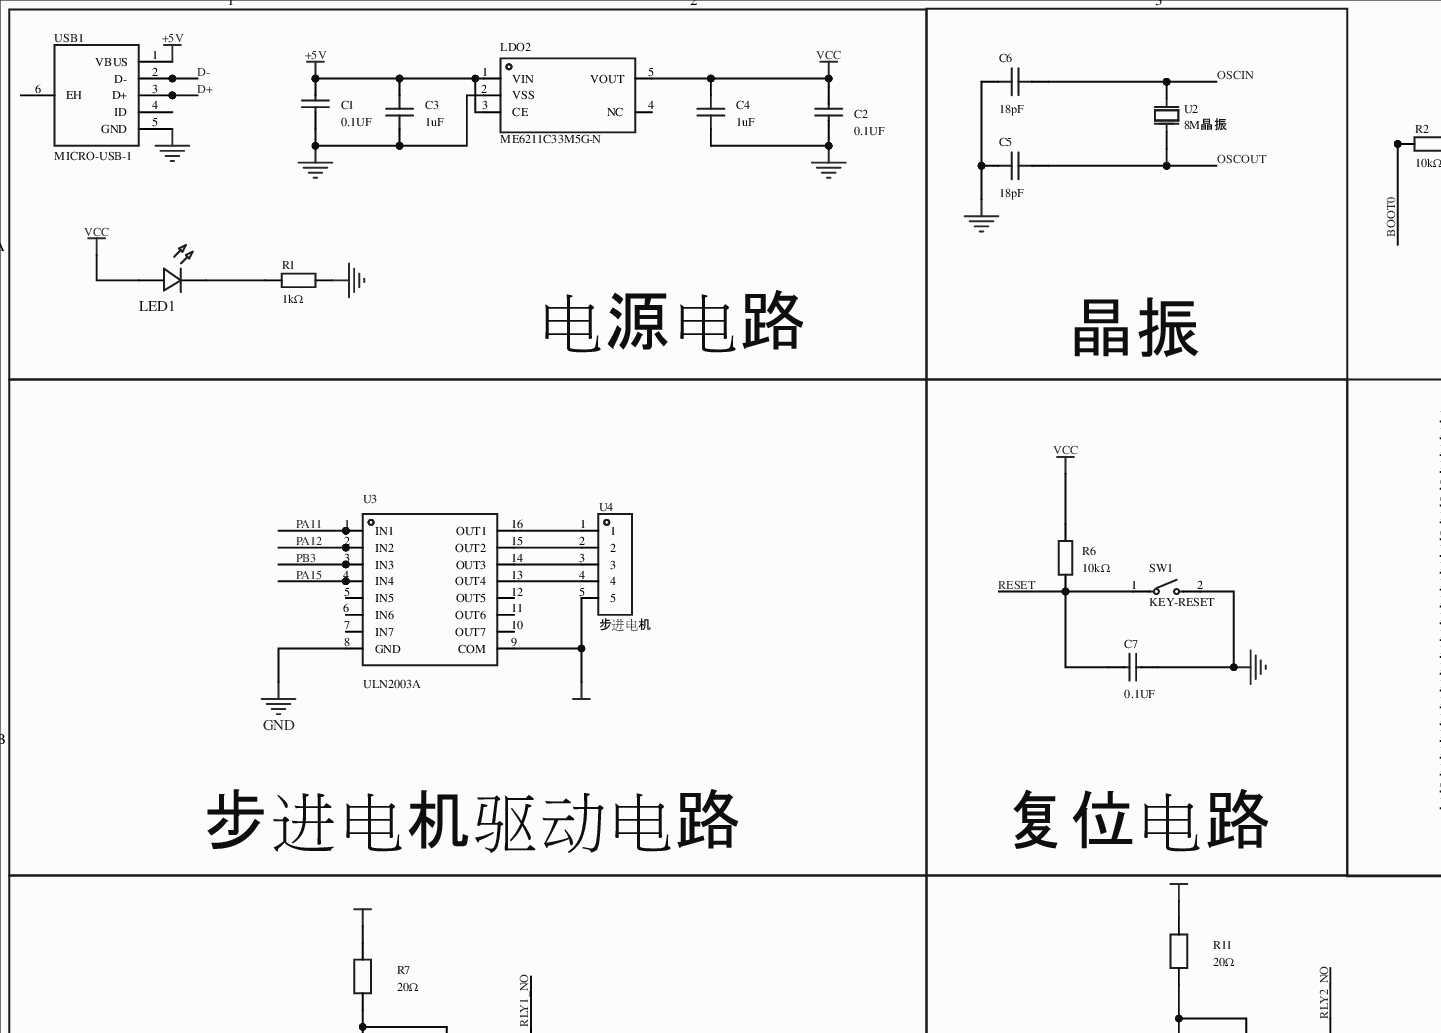
[diagram p0: MISC51317-3.schdoc, top left]
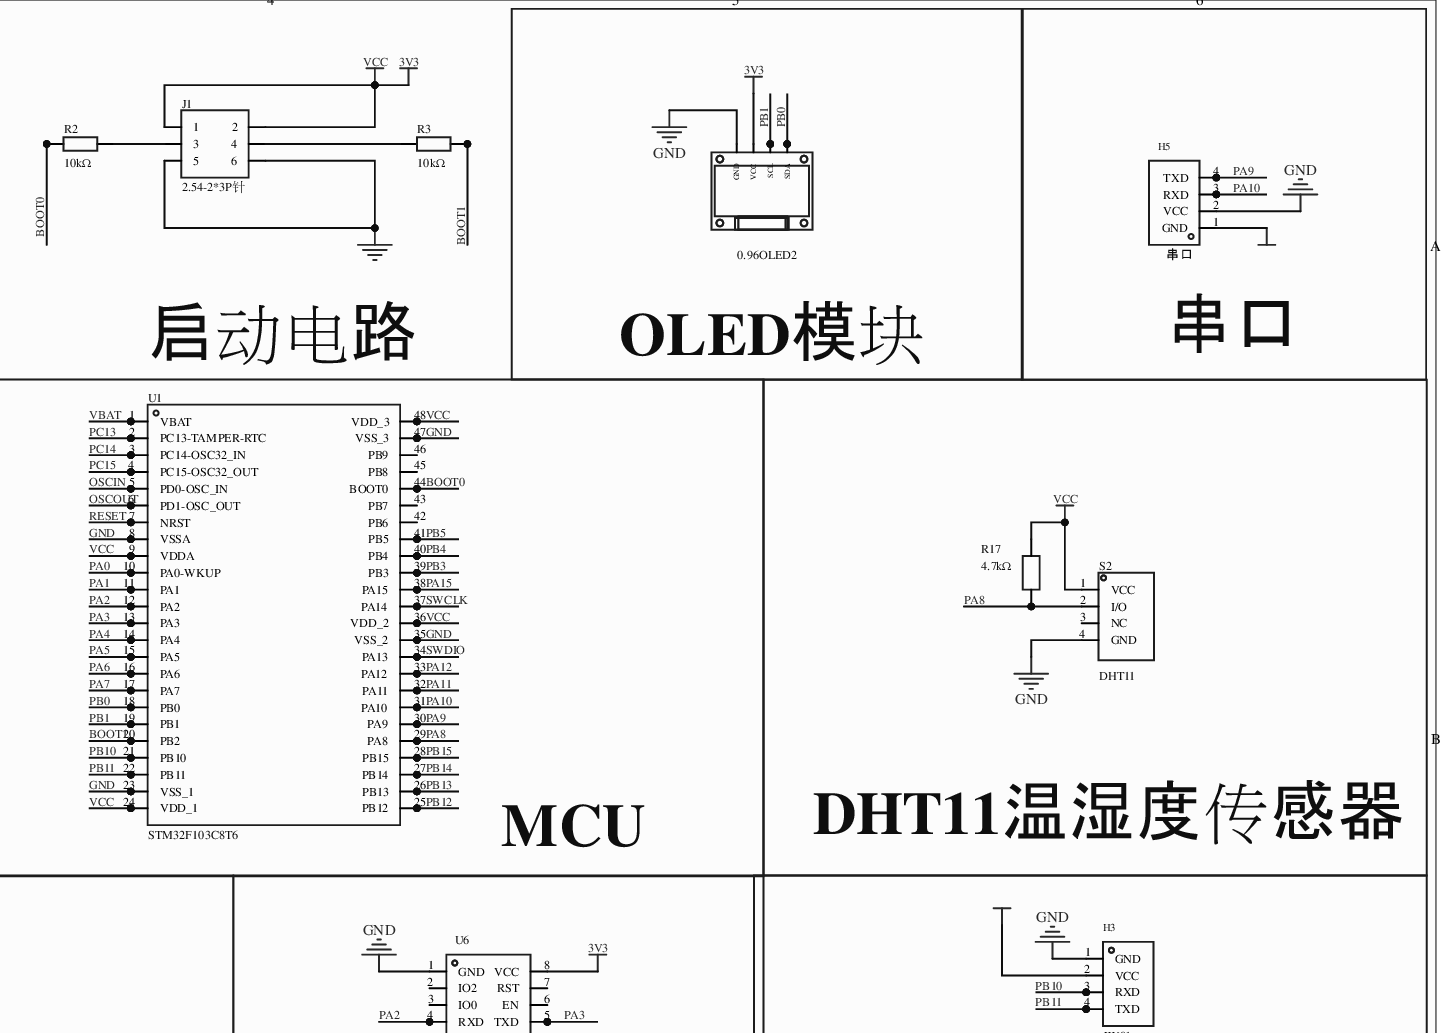
[diagram p1: MISC51317-3.schdoc, top right]
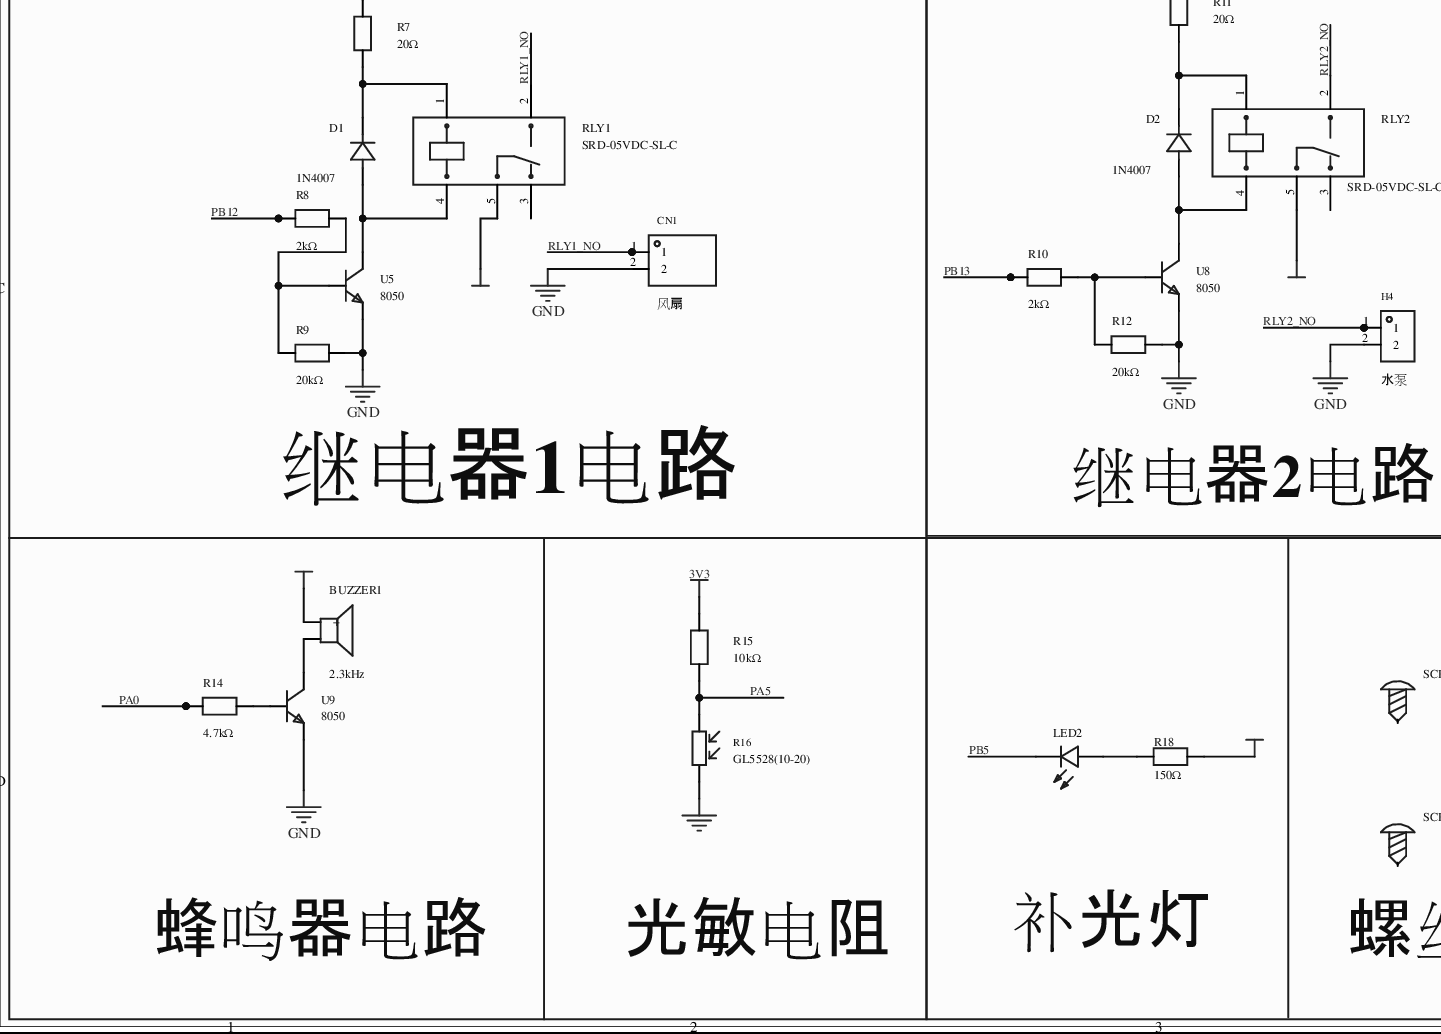
[diagram p2: MISC51317-3.schdoc, bottom left]
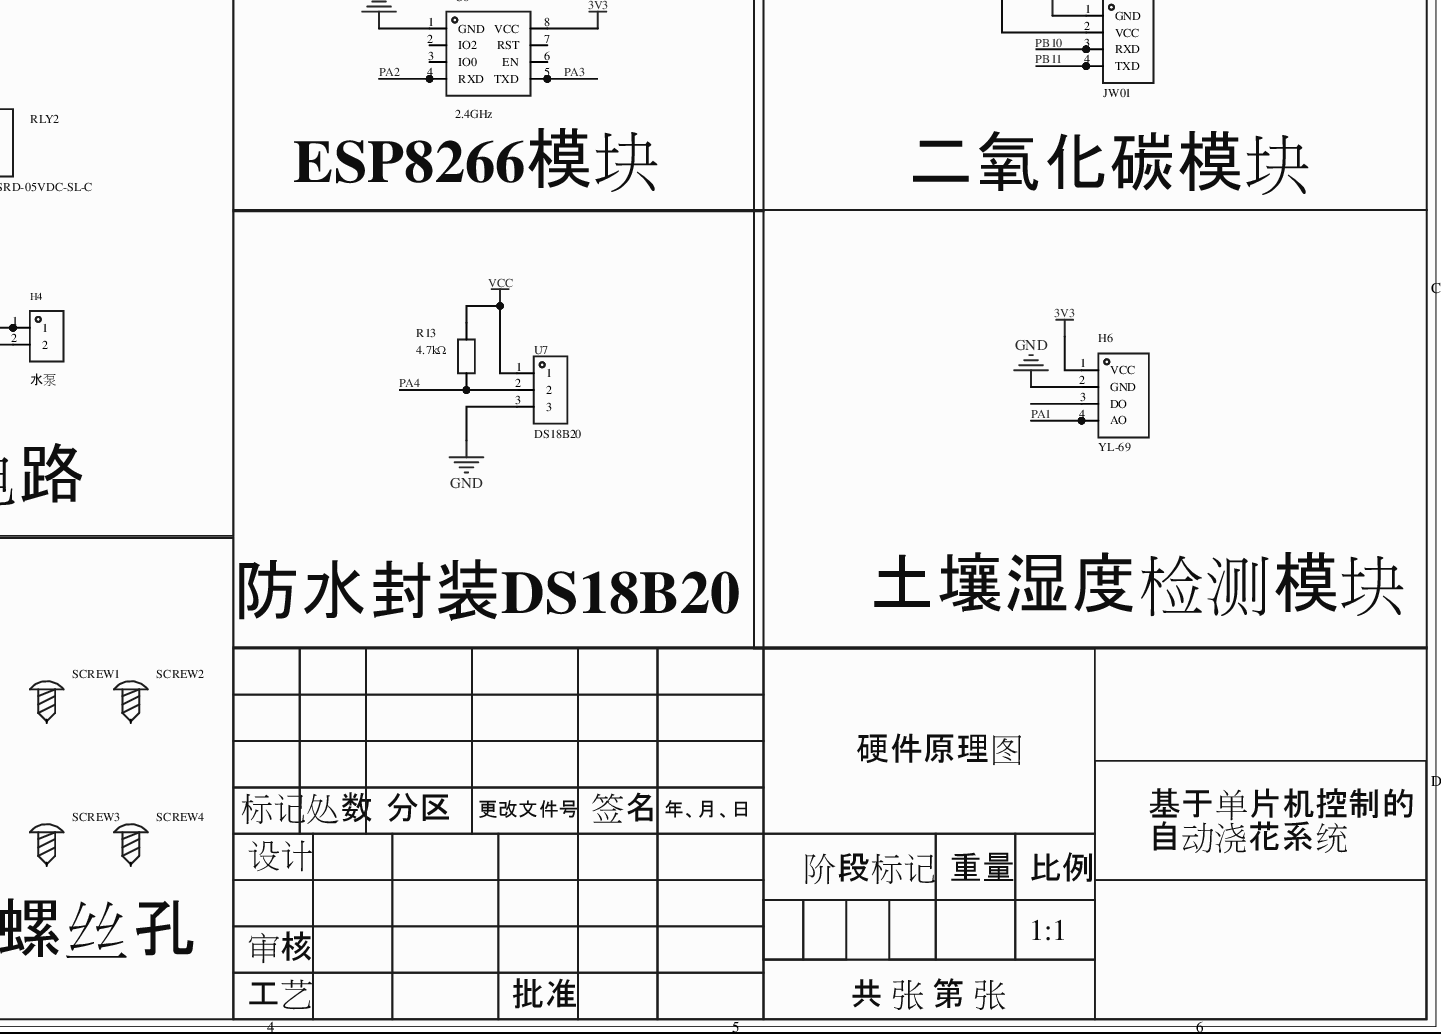
[diagram p3: MISC51317-3.schdoc, bottom right]
# Altium project MISC51317-2.PrjPcb
1 sheet, 54 parts. Net scope: global (net labels, ports and power ports of the same name join across sheets).
Board file: MISC51317.pcbdoc

## Sheet MISC51317-3.schdoc
size 420 x 297 mm; Version: V1.0; @Project Name: MISC51317; @Update Date: 2026-04-15; @Create Date: 2026-04-15; @Board Name: MISC51317; @Create Time: 10:52:34; @Page Count: 1; @Page No: 1; @Schematic Name: MISC51317; @Update Time: 10:52:34; Size: A4

### Parts
0.96OLED2  (no value)  [oled-th_l27.8-w27.2-p2.54_c9900033791]
BUZZER1  2.3kHz  [BUZ-TH_BD12.0-P7.60-D0.6-FD]
C1  0.1UF  [C0603]
C2  0.1UF  [C0603]
C3  1uF  [C0603]
C4  1uF  [C0603]
C5  18pF  [C0603]
C6  18pF  [C0603]
C7  0.1UF  [C0603]
CN1  风扇  [CONN-TH_B2B-XH-A-LF-SN]
D1  1N4007  [DO-41_BD2.4-L4.7-P8.70-D0.8-RD]
D2  1N4007  [DO-41_BD2.4-L4.7-P8.70-D0.8-RD]
H3  JW01  [HDR-TH_4P-P2.54-V-M]
H4  水泵  [HDR-TH_2P-P2.54-V-M]
H5  串口  [HDR-TH_4P-P2.54-V-M]
H6  YL-69  [HDR-TH_4P-P2.54-V-F]
J1  2.54-2*3P针  [HDR-TH_6P-P2.54-V-M-R2-C3-S2.54-1]
LDO2  ME6211C33M5G-N  [SOT-23-5_L3.0-W1.7-P0.95-LS2.8-BL]
LED1  (no value)  [LED_0603]
LED2  (no value)  [LED-TH_BD5.9-P2.54-RD]
R1  1kΩ  [R0603]
R2  10kΩ  [R0603]
R3  10kΩ  [R0603]
R6  10kΩ  [R0603]
R7  20Ω  [RES-TH_BD2.3-L6.5-P10.50-D0.5]
R8  2kΩ  [RES-TH_BD2.3-L6.5-P10.50-D0.5]
R9  20kΩ  [RES-TH_BD2.3-L6.5-P10.50-D0.5]
R10  2kΩ  [RES-TH_BD2.3-L6.5-P10.50-D0.5]
R11  20Ω  [RES-TH_BD2.3-L6.5-P10.50-D0.5]
R12  20kΩ  [RES-TH_BD2.3-L6.5-P10.50-D0.5]
R13  4.7kΩ  [RES-TH_BD2.3-L6.5-P10.50-D0.5]
R14  4.7kΩ  [RES-TH_BD2.3-L6.5-P10.50-D0.5]
R15  10kΩ  [RES-TH_BD2.3-L6.5-P10.50-D0.5]
R16  GL5528(10-20)  [RES-TH_L5.1-W4.3-P3.40-D0.5]
R17  4.7kΩ  [RES-TH_BD2.3-L6.5-P10.50-D0.5]
R18  150Ω  [RES-TH_BD2.3-L6.5-P10.50-D0.5]
RLY1  SRD-05VDC-SL-C  [RELAY-TH_SRD-XXVDC-XL-C]
RLY2  SRD-05VDC-SL-C  [RELAY-TH_SRD-XXVDC-XL-C]
S2  DHT11  [SENSOR-TH_DHT11-1]
SCREW1  (no value)  [M2螺丝]
SCREW2  (no value)  [M2螺丝]
SCREW3  (no value)  [M2螺丝]
SCREW4  (no value)  [M2螺丝]
SW1  KEY-RESET  [SW-SMD_L6.0-W3.3-LS8.0]
U1  STM32F103C8T6  [LQFP-48_L7.0-W7.0-P0.50-LS9.0-BL]
U2  8M晶振  [HC-49S_L11.5-W4.7-P4.88]
U3  ULN2003A  [DIP-16_L20.0-W6.4-P2.54-LS7.6-BL]
U4  步进电机  [CONN-TH_5P-P2.50_ZHOURI_XH-5PA]
U5  8050  [TO-92-3_L4.8-W3.7-P2.54-R]
U6  2.4GHz  [WIFIM-TH_8P-L24.7-W14.4-P2.54]
U7  DS18B20  [CONN-TH_3P-P5.00_KF301-5.0-3P]
U8  8050  [TO-92-3_L4.8-W3.7-P2.54-R]
U9  8050  [TO-92-3_L4.8-W3.7-P2.54-R]
USB1  MICRO-USB-1  [MICRO-USB-SMD_C9900008946]

### Blocks framed on the sheet
电源电路: C1-C4 LDO2 LED1 R1 USB1
晶振: C5 C6 U2
OLED模块: 0.96OLED2
串口: H5
步进电机驱动电路: U3 U4
复位电路: C7 R6 SW1
DHT11温湿度传感器: R17 S2
继电器1电路: CN1 D1 R7-R9 RLY1 U5
继电器2电路: D2 H4 R10-R12 RLY2 U8
二氧化碳模块: H3
土壤湿度检测模块: H6
蜂鸣器电路: BUZZER1 R14 U9
光敏电阻: R15 R16

### Nets
+5V: C1.2 C3.2 LDO2.1(VIN) LDO2.3(CE) USB1.1(VBUS)
GND: 0.96OLED2.1(GND) C1.1 C2.1 C3.1 C4.1 C5.2 C6.1 C7.2 CN1.2 H3.1(GND) H4.2 H5.2(VCC) H6.2(GND) J1.5 J1.6 LDO2.2(VSS) R1.2 R9.2 R12.2 R16.2 S2.4(GND) SW1.2 U1.8(VSSA) U1.23(VSS_1) U1.35(VSS_2) U1.47(VSS_3) U3.8(GND) U5.3(E) U6.1(GND) U7.3 U8.3(E) U9.3(E) USB1.5(GND)
3V3: 0.96OLED2.2(VCC) BUZZER1.1(+) C2.2 C4.2 H3.2(VCC) H5.1(GND) H6.1(VCC) J1.1 J1.2 LDO2.5(VOUT) LED1.2(A) R6.2 R7.2 R11.2 R13.2 R15.2 R17.2 R18.2 RLY1.5 RLY2.5 S2.1(VCC) U1.9(VDDA) U1.24(VDD_1) U1.36(VDD_2) U1.48(VDD_3) U3.9(COM) U4.5 U6.8(VCC) U7.1  [also labelled VCC]
BOOT0: R2.1 U1.44(BOOT0)
BOOT1: R3.2 U1.20(PB2)
D+: USB1.3(D+)
D-: USB1.2(D-)
OSCIN: C6.2 U1.5(PD0-OSC_IN) U2.1(OSC1)
OSCOUT: C5.1 U1.6(PD1-OSC_OUT) U2.2(OSC2)
PA0: R14.1 U1.10(PA0-WKUP)
PA1: H6.4(AO) U1.11(PA1)
PA2: U1.12(PA2) U6.4(RXD)
PA3: U1.13(PA3) U6.5(TXD)
PA4: R13.1 U1.14(PA4) U7.2
PA5: R15.1 R16.1 U1.15(PA5)
PA6: U1.16(PA6)
PA7: U1.17(PA7)
PA8: R17.1 S2.2(I/O) U1.29(PA8)
PA9: H5.4(TXD) U1.30(PA9)
PA10: H5.3(RXD) U1.31(PA10)
PA11: U1.32(PA11) U3.1(IN1)
PA12: U1.33(PA12) U3.2(IN2)
PA15: U1.38(PA15) U3.4(IN4)
PB0: 0.96OLED2.4(SDA) U1.18(PB0)
PB1: 0.96OLED2.3(SCL) U1.19(PB1)
PB3: U1.39(PB3) U3.3(IN3)
PB4: U1.40(PB4)
PB5: LED2.1(C) U1.41(PB5)
PB10: H3.3(RXD) U1.21(PB10)
PB11: H3.4(TXD) U1.22(PB11)
PB12: R8.1 U1.25(PB12)
PB13: R10.1 U1.26(PB13)
PB14: U1.27(PB14)
PB15: U1.28(PB15)
PC13: U1.2(PC13-TAMPER-RTC)
PC14: U1.3(PC14-OSC32_IN)
PC15: U1.4(PC15-OSC32_OUT)
RESET: C7.1 R6.1 SW1.1 U1.7(NRST)
RLY1_NO: CN1.1 RLY1.2
RLY2_NO: H4.1 RLY2.2
SWCLK: U1.37(PA14)
SWDIO: U1.34(PA13)
VBAT: U1.1(VBAT)
NetBUZZER1_2: BUZZER1.2 U9.1(C)
NetD1_1: D1.1(K) R7.1 RLY1.1
NetD1_2: D1.2(A) RLY1.4 U5.1(C)
NetD2_1: D2.1(K) R11.1 RLY2.1
NetD2_2: D2.2(A) RLY2.4 U8.1(C)
NetJ1_3: J1.3 R2.2
NetJ1_4: J1.4 R3.1
NetLED1_1: LED1.1(C) R1.1
NetLED2_2: LED2.2(A) R18.1
NetR8_2: R8.2 R9.1 U5.2(B)
NetR10_2: R10.2 R12.1 U8.2(B)
NetR14_2: R14.2 U9.2(B)
NetU3_13: U3.13(OUT4) U4.4
NetU3_14: U3.14(OUT3) U4.3
NetU3_15: U3.15(OUT2) U4.2
NetU3_16: U3.16(OUT1) U4.1

Not connected (* = marked no-connect by the designer): H6 3(DO); LDO2 4(NC)*; RLY1 3*; RLY2 3*; S2 3(NC); SCREW1 1; SCREW2 1; SCREW3 1; SCREW4 1; U1 42(PB6)* 43(PB7)* 45(PB8)* 46(PB9)*; U3 5(IN5)* 6(IN6)* 7(IN7)* 10(OUT7)* 11(OUT6)* 12(OUT5)*; U6 2(IO2)* 3(IO0)* 6(EN)* 7(RST)*; USB1 4(ID)* 6(EH)*

### Notes on the sheet
- (near U1) 启动电路
- MCU
- (near U6) ESP8266模块
- 防水封装DS18B20
- 硬件原理图
- 基于单片机控制的
  自动浇花系统
- 标记
- 设计
- 处数
- 分区
- 更改文件号
- 签名
- 年、月、日
- 阶段标记
- 重量
- 比例
- 补光灯
- 螺丝孔
- 审核
- 1:1
- 工艺
- 批准
- 共 张 第 张

### Library data of the parts
0.96OLED2 = 0.96OLED模块_4P: 3D Model: 79c000fdb68d45a296c2e9bedf4f9055; 3D Model Transform: 1393.69792,1318.895,0,0,0,0,0,-560.079,-137.795; ConvertToPcb: yes; ModelName: 0.96OLED_4P; Device: 0.96OLED模块_4P; Symbol: 0.96OLED模块_4P; Supplier Footprint: 插件; FootprintName: oled-th_l27.8-w27.2-p2.54_c9900033791; AddInBom: yes
BUZZER1 = TMB12A05_C96093: 驱动方式:有源(内含驱动线路);构造类型:电磁式;额定电压:5V;频率:2.3kHz;声压(SPL):85dB@5V,10cm;; Manufacturer: 华能; 3D Model: 16ab50e14c5b4f2c986c135bdba60e37; 3D Model Transform: 472.44,472.176,0,90,0,0,-0.787,0,-177.165; Technology Type: 电磁式; Rated Voltage: 5V; Operating Voltage: 4V~8V; AddInBom: yes; ModelName: BUZ-TH_D12.0-H9.5-P7.60; Device: TMB12A05_C96093; Symbol: TMB12A05; LCSC Part Name: TMB12A05; Supplier Part: C96093; Manufacturer Part: TMB12A05; Supplier Footprint: 插件,D=12mm; JLCPCB Part Class: Extended Part; Datasheet: https://atta.szlcsc.com/upload/public/pdf/source/20170522/1495448324811.pdf; Supplier: LCSC; Oscillator Circuit: 有源(内含驱动线路); Value: 2.3kHz; Sound Pressure Level (SPL): 85dB@5V,10cm; Diameter (φD): 12mm; Height: 9.8mm; FootprintName: BUZ-TH_BD12.0-P7.60-D0.6-FD; ConvertToPcb: yes
C1 C2 = CAPCER0.1UF16VX5R0603,CAPCER0.1UF25VX5R0603,CAPCER0.1UF16VX7R0603: AddInBom: yes; ModelId: ac125912035d415993ca9572d50418b10819f05c4eef4c71ace90d822a990e87; ModelName: C0603_L1.6-W0.8-H0.8; ModelTransform: 62.992,31.496,0,0,0,0,0,0,0; Device: CAPCER0.1UF16VX5R0603,CAPCER0.1UF25VX5R0603,CAPCER0.1UF16VX7R0603; Symbol: CAPCER0.1UF16VX5R0603,CAPCER0.1UF25VX5R0603,CAPCER0.1UF16VX7R0603; Manufacturer Part: 0.1UF; FootprintName: C0603; LCSC Part Name: CAPCER0.1UF16VX5R0603,CAPCER0.1UF25VX5R0603,CAPCER0.1UF16VX7R0603; SupplierPart: C9900012833; Supplier Footprint: C0603; JLCPCB Part Class: Extended Part; Supplier: LCSC; ConvertToPcb: yes
C3 C4 = TMK107B7105MA-T: 容值:1uF;精度:±20%;额定电压:25V;温度系数:X7R;; Manufacturer: TAIYO YUDEN(太诱); AddInBom: yes; Tolerance: ±20%; Voltage Rating: 25V; Temperature Coefficient: X7R; ModelId: ac125912035d415993ca9572d50418b10819f05c4eef4c71ace90d822a990e87; ModelName: C0603_L1.6-W0.8-H0.8; ModelTransform: 62.992,31.496,0,0,0,0,0,0,0; Device: TMK107B7105MA-T; Symbol: TMK107B7105MA-T; FootprintName: C0603; LCSC Part Name: MSAST168SB7105MTNA01 1uF ±20% 25V; SupplierPart: C2180866; ManufacturerPart: TMK107B7105MA-T; Supplier Footprint: 0603; JLCPCB Part Class: Extended Part; Datasheet: https://item.szlcsc.com/datasheet/TMK107B7105MA-T/2272933.html; Supplier: LCSC; ConvertToPcb: yes; Value: 1uF
C5 C6 = C1608C0G1H180J080AA: 容值:18pF;精度:±5%;额定电压:50V;材质(温度系数):C0G;; Manufacturer: TDK; AddInBom: yes; Tolerance: ±5%; Voltage Rated: 50V; Temperature Coefficient: C0G; ModelId: ac125912035d415993ca9572d50418b10819f05c4eef4c71ace90d822a990e87; ModelName: C0603_L1.6-W0.8-H0.8; ModelTransform: 62.992,31.496,0,0,0,0,0,0,0; Device: C1608C0G1H180J080AA; Symbol: C1608C0G1H180J080AA; FootprintName: C0603; LCSC Part Name: 18pF ±5% 50V; SupplierPart: C3902597; ManufacturerPart: C1608C0G1H180J080AA; Supplier Footprint: 0603; JLCPCB Part Class: Extended Part; Datasheet: https://atta.szlcsc.com/upload/public/pdf/source/20230606/A83975C7E70EF5AFCD4A17254ABD78F2.pdf; Supplier: LCSC; ConvertToPcb: yes; Value: 18pF
C7 = CAPCER0.1UF16VX5R0603,CAPCER0.1UF25VX5R0603,CAPCER0.1UF16VX7R0603: 3D Model: ac125912035d415993ca9572d50418b10819f05c4eef4c71ace90d822a990e87; 3D Model Transform: 62.992,31.496,0,0,0,0,0,0,0; AddInBom: yes; ModelName: C0603_L1.6-W0.8-H0.8; Device: CAPCER0.1UF16VX5R0603,CAPCER0.1UF25VX5R0603,CAPCER0.1UF16VX7R0603; Symbol: CAPCER0.1UF16VX5R0603,CAPCER0.1UF25VX5R0603,CAPCER0.1UF16VX7R0603; LCSC Part Name: CAPCER0.1UF16VX5R0603,CAPCER0.1UF25VX5R0603,CAPCER0.1UF16VX7R0603; Supplier Part: C9900012833; Manufacturer Part: 0.1UF; Supplier Footprint: C0603; JLCPCB Part Class: Extended Part; Supplier: LCSC; FootprintName: C0603; ConvertToPcb: yes
CN1 = B2B-XH-A(LF)(SN): 参考系列:XH;间距:2.5mm;插针结构:1x2P;排数:1;每排PIN数:2;行距:-;安装方式:-;触头材质:黄铜;; Manufacturer: JST; 3D Model: 2cd591bdb98c4759a6cba2f4f7745e41; 3D Model Transform: 295.275,224.44837,0,180,0,0,0,18.701,-98.425; Reference Series: XH; Pitch: 2.5mm; Pins Structure: 1x2P; Number of PINs Per Row: 2; AddInBom: yes; ModelName: XH2.5-2A; Device: B2B-XH-A(LF)(SN); Symbol: B2B-XH-A (LF)(SN); Manufacturer Part: 风扇; LCSC Part Name: 系列:XH 间距:2.5mm 1x2P; Supplier Footprint: 插件,P=2.5mm; Datasheet: https://atta.szlcsc.com/upload/public/pdf/source/20180928/C265283_F9DFEEBDB2CF642B6BDFAB4B77BD2680.pdf; Number of Rows: 1; Row Spacing: -; Mounting Style: -; Contact Material: 黄铜; Supplier: LCSC; Supplier Part: C158012; JLCPCB Part Class: 扩展库; FootprintName: CONN-TH_B2B-XH-A-LF-SN; ConvertToPcb: yes
D1 D2 = 1N4007_C2985028: 直流反向耐压(Vr):1kV;平均整流电流(Io):1A;正向压降(Vf):1V@1A;; Manufacturer: GOODWORK(固得沃克); 3D Model: 6de1e9b71a0d4751b4e9df530304c1a3; 3D Model Transform: 374.015,94.428,0,0,0,0,0,0,-137.795; Reverse Voltage (Vr): 1kV; Average Rectified Current (Io): 1A; Forward Voltage (Vf@If): 1V@1A; AddInBom: yes; ModelName: DO-41_D2.4-L4.7-P8.70; Device: 1N4007_C2985028; Symbol: 1N4007_C2985028; LCSC Part Name: 1kV 1A 1V@1A; Supplier Part: C2985028; Manufacturer Part: 1N4007; Supplier Footprint: DO-41; JLCPCB Part Class: 扩展库; Datasheet: https://atta.szlcsc.com/upload/public/pdf/source/20210723/C2848669_ECFE0BC1B34B7BAAA686846FF0F306A7.pdf; Supplier: LCSC; FootprintName: DO-41_BD2.4-L4.7-P8.70-D0.8-RD; ConvertToPcb: yes
H3 H5 = PZ254V-11-04P: 排数:单排;总PIN位数:4P;间距:2.54mm;插针结构:1x4P;行距:-;安装类型:直插;圆针/方针:方针;额定电流:3A;额定电压:250V;配合针长度:6mm;塑高:2.5mm;端接针长度:3mm;触头材质:-;工作温度范围:-40℃~+105℃;颜色:黑色;; Manufacturer: XFCN(兴飞); Symbol: PZ254V-11-04P_C2691448; 3D Model: 112f4d05e8d64e99ab9a333894bea4f9; 3D Model Transform: 399.999,104.7242,0,0,0,0,0,0,-118.11; Pitch: 2.54mm; Pin Structure: 1x4P; Circluar Pins/Square Pins: 方针; Current Rating (Max): 3A; Voltage Rating (Max): 250V; AddInBom: yes; ModelName: HDR-TH_4P-P2.54-M-LI-1X4P; Device: PZ254V-11-04P; LCSC Part Name: 2.54mm 1x4P 直插 方针; Supplier Part: C2691448; Supplier Footprint: 插件,P=2.54mm; JLCPCB Part Class: 扩展库; Datasheet: https://atta.szlcsc.com/upload/public/pdf/source/20200309/C492403_F9F19131791D08044AD4F84F8E751A34.pdf; Supplier: LCSC; Number of Rows: 单排; Number of Pins: 4P; Row Spacing: -; Mounting Type: 直插; Length of Mating Pin: 6mm; Insulation Height: 2.5mm; Length of End Connection Pin: 3mm; Contact Material: -; Operating Temperature Range: -40℃~+105℃; Color: 黑色; FootprintName: HDR-TH_4P-P2.54-V-M; ConvertToPcb: yes
  H3: Manufacturer Part: JW01
  H5: Manufacturer Part: 串口
H4 = PZ254V-11-02P: 排数:单排;总PIN位数:2P;间距:2.54mm;插针结构:1x2P;行距:-;安装类型:直插;圆针/方针:方针;额定电流:-;额定电压:-;配合针长度:6mm;塑高:2.5mm;端接针长度:3mm;触头材质:黄铜;触头镀层:-;工作温度范围:-40℃~+105℃;颜色:黑色;; Manufacturer: XFCN(兴飞); 3D Model: e35305ec3aa84b66b849f914b715e73f; 3D Model Transform: 200,100,0,0,0,0,0,0,-118.11; Pitch: 2.54mm; Pin Structure: 1x2P; Circluar Pins/Square Pins: 方针; AddInBom: yes; ModelName: HDR2.54-M-LI-1X2P; Device: PZ254V-11-02P; Symbol: PZ254V-11-02P; Manufacturer Part: 水泵; LCSC Part Name: 2.54mm 1x2P 直插 方针; Supplier Footprint: 插件,P=2.54mm; Datasheet: https://atta.szlcsc.com/upload/public/pdf/source/20200309/C492401_A812433581A9B211A7FFA413ADDFF0E5.pdf; Number of Rows: 单排; Number of Pins: 2P; Row Spacing: -; Mounting Type: 直插; Current Rating (Max): -; Voltage Rating (Max): -; Length of Mating Pin: 6mm; Insulation Height: 2.5mm; Length of End Connection Pin: 3mm; Contact Material: 黄铜; Contact Plating: -; Operating Temperature Range: -40℃~+105℃; Color: 黑色; Supplier: LCSC; Supplier Part: C492401; JLCPCB Part Class: 扩展库; FootprintName: HDR-TH_2P-P2.54-V-M; ConvertToPcb: yes
H6 = PM254V-11-04-H85: 排数:单排;总孔位数:4P;间距:2.54mm;插孔结构:1x4P;行距:-;安装类型:直插;塑高:-;触头材质:黄铜;触头镀层:-;; Manufacturer: XFCN(兴飞); 3D Model: 57daaad411c24bd7bd5d06edf5c4d16b; 3D Model Transform: 415.7472,98.425,0,0,0,0,0,0,-118.11; Number of Holes: 4P; Pitch: 2.54mm; Holes Structure: 1x4P; AddInBom: yes; ModelName: HDR-TH_4P-P2.54-F-LI-1X4P; Device: PM254V-11-04-H85; Symbol: PM254V-11-04-H85; Manufacturer Part: YL-69; LCSC Part Name: 间距:2.54mm 1x4P 直插; Supplier Part: C541851; Supplier Footprint: 插件,P=2.54mm; JLCPCB Part Class: 扩展库; Datasheet: https://atta.szlcsc.com/upload/public/pdf/source/20200518/C541849_85853D71FC67C51915A806977A588FDA.pdf; Supplier: LCSC; Number of Rows: 单排; Row Spacing: -; Mounting Type: 直插; Insulation Height: -; Contact Material: 黄铜; Contact Plating: -; FootprintName: HDR-TH_4P-P2.54-V-F; ConvertToPcb: yes
J1 = 2.54-2*3P针: 插针结构:-;间距:2.54mm;行距:2.54mm;圆针/方针:-;安装方式:直插;排数:双排;总PIN位数:6P;额定电流:-;额定电压:-;配合针长度:-;塑高:-;触头材质:-;触头镀层:-;颜色:黑色;; Manufacturer: BOOMELE(博穆精密); Symbol: Header-Male-2.54_2x3; AddInBom: yes; Pitch: 2.54mm; ModelId: fd1b55b786fb415ca65c4187088147b70819f05c4eef4c71ace90d822a990e87; ModelName: HDR2.54-M-LI-2x3P; ModelTransform: 299.9994,200,0,0,0,0,0,0,-118.11; Device: 2.54-2*3P针; FootprintName: HDR-TH_6P-P2.54-V-M-R2-C3-S2.54-1; LCSC Part Name: 间距:2.54mm 直插; SupplierPart: C65114; ManufacturerPart: 2.54-2*3P针; Supplier Footprint: 插件,P=2.54mm; JLCPCB Part Class: Extended Part; Supplier: LCSC; ConvertToPcb: yes; Pin Structure: -; Row Spacing: 2.54mm; Circluar Pins/Square Pins: -; Mounting Type: 直插; Number of Rows: 双排; Number of Pins: 6P; Current Rating: -; Voltage Rating (Max): -; Length of Mating Pin: -; Insulation Height: -; Contact Material: -; Contact Plating: -; Color: 黑色
LDO2 = ME6211C33M5G-N: 输出类型:固定;工作电压:6V;输出电压:3.3V;输出电流:500mA;电源纹波抑制比(PSRR):70dB@(1kHz);输出极性:正极;; Manufacturer: MICRONE(南京微盟); AddInBom: yes; Output Type: 固定; Voltage - Supply: 6V; Output Voltage: 3.3V; Output Current: 500mA; Voltage Dropout: 120mV@(100mA); standby current: 60uA; Noise: 50uVrms; Output Configuration: 正极; Number of Outputs: 1; ModelId: 0a2a1b8f50944f73965918ad6e5fe1670819f05c4eef4c71ace90d822a990e87; ModelName: SOT-23-5_L2.9-W1.6-H1.1-LS2.8-P0.95; ModelTransform: 118.60433,114.173,0,90,0,0,0.0005,0.0005,0; Device: ME6211C33M5G-N; Symbol: ME6211C33M5G-N; FootprintName: SOT-23-5_L3.0-W1.7-P0.95-LS2.8-BL; LCSC Part Name: 输入6V 输出3.3V 500mA; SupplierPart: C82942; ManufacturerPart: ME6211C33M5G-N; Supplier Footprint: SOT-23-5; JLCPCB Part Class: Extended Part; Datasheet: https://item.szlcsc.com/datasheet/ME6211C33M5G-N/84106.html; Supplier: LCSC; ConvertToPcb: yes; Power Supply Rejection Ratio (PSRR): 70dB@(1kHz); Features: 过流保护；带使能；短路保护; Operating Temperature: -40℃~+150℃
LED1 = LED_0603-R: Symbol: LED_R; Convert to PCB: yes; 3D Model: dd8257b0d61a4cd7b68939a056e080950819f05c4eef4c71ace90d822a990e87; 3D Model Transform: 58.72,29.4,22.03,0,0,0,0,0,0; ModelName: LED-0603_R; Device: LED_0603-R; Add into BOM: yes; Supplier Footprint: 0603; FootprintName: LED_0603
LED2 = 333-2SURD/S530-A3: 发光颜色:红灯;; Manufacturer: EVERLIGHT(亿光); 3D Model: 0ecbca0d139a466b8fc3aef618bbaa4e; 3D Model Transform: 211.96686,228.01584,0,0,0,0,7.874,0,-137.795; Emitted Color: 红灯; Lamp Holder Type: 5mm圆形灯头; AddInBom: yes; Device: 333-2SURD/S530-A3; Symbol: 333-2SURD/S530-A3; LCSC Part Name: 红灯; Supplier Part: C87271; Supplier Footprint: 插件,D=5mm; JLCPCB Part Class: 扩展库; Datasheet: https://atta.szlcsc.com/upload/public/pdf/source/20161119/1479540195109.pdf; Supplier: LCSC; FootprintName: LED-TH_BD5.9-P2.54-RD; ConvertToPcb: yes; ModelName: LED-TH_BD5.9-P2.54-RD
R1 = 0603WAF1001T5E: 电阻类型:厚膜电阻;阻值:1kΩ;精度:±1%;功率:100mW;工作电压:75V;温度系数:±100ppm/℃;; Manufacturer: UNI-ROYAL(厚声); AddInBom: yes; Tolerance: ±1%; Power(Watts): 100mW; Voltage-Supply(Max): 75V; ModelId: fc143cca1e79419f9cd78b61e9279f080819f05c4eef4c71ace90d822a990e87; ModelTransform: 31.8897,63.7794,0,90,0,0,0,0,0; Device: 0603WAF1001T5E; Symbol: 0603WAF1001T5E; FootprintName: R0603; LCSC Part Name: 1kΩ ±1% 100mW 厚膜电阻; SupplierPart: C21190; ManufacturerPart: 0603WAF1001T5E; Supplier Footprint: 0603; JLCPCB Part Class: Basic Part; Datasheet: https://item.szlcsc.com/datasheet/0603WAF1001T5E/21904.html; Supplier: LCSC; ConvertToPcb: yes; Type: 厚膜电阻; Value: 1kΩ; Temperature Coefficient: ±100ppm/℃; Operating Temperature: -55℃~+155℃; ModelName: R0603
R2 R3 R6 = 0603WAF1002T5E: 电阻类型:厚膜电阻;阻值:10kΩ;精度:±1%;功率:100mW;工作电压:75V;温度系数:±100ppm/℃;; Manufacturer: UNI-ROYAL(厚声); AddInBom: yes; Tolerance: ±1%; Power(Watts): 100mW; Voltage-Supply(Max): 75V; ModelId: fc143cca1e79419f9cd78b61e9279f080819f05c4eef4c71ace90d822a990e87; ModelTransform: 31.8897,63.7794,0,90,0,0,0,0,0; Device: 0603WAF1002T5E; Symbol: 0603WAF1002T5E; FootprintName: R0603; LCSC Part Name: 厚膜电阻 10kΩ ±1% 100mW; SupplierPart: C25804; ManufacturerPart: 0603WAF1002T5E; Supplier Footprint: 0603; JLCPCB Part Class: Basic Part; Datasheet: https://item.szlcsc.com/datasheet/0603WAF1002T5E/26547.html; Supplier: LCSC; ConvertToPcb: yes; Type: 厚膜电阻; Value: 10kΩ; Temperature Coefficient: ±100ppm/℃; Operating Temperature: -55℃~+155℃; ModelName: R0603
R7-R15 R17 R18 = MF1/4W-1KΩ±1%T52: 电阻类型:金属膜电阻;阻值:1kΩ;精度:±1%;功率:250mW;温度系数:±200ppm/℃;; Manufacturer: 华星机电; 3D Model: 8e6c7ee8323443d1ab8f0504b6353c8c; 3D Model Transform: 431.1015,91.3384,0,0,0,0,0.197,0,-137.795; Tolerance: ±1%; Power(Watts): 250mW; AddInBom: yes; ModelName: RES-TH_D2.3-L6.5-P10.50; Device: MF1/4W-1KΩ±1%T52; Symbol: MF1/4W-1KΩ±1%T52; LCSC Part Name: 1kΩ ±1% 250mW; Manufacturer Part: MF1/4W-1KΩ±1%T52; Supplier Footprint: 轴向引线; JLCPCB Part Class: 扩展库; Datasheet: https://atta.szlcsc.com/upload/public/pdf/source/20200731/C713882_AE8EB1102749D7E4FB4FB13DC898C429.pdf; Supplier: LCSC; Type: 金属膜电阻; Temperature Coefficient: ±200ppm/℃; FootprintName: RES-TH_BD2.3-L6.5-P10.50-D0.5; ConvertToPcb: yes
  R7 R11: Value: 20Ω
  R8 R10: Value: 2kΩ
  R9 R12: Value: 20kΩ
  R13 R14 R17: Value: 4.7kΩ
  R15: Value: 10kΩ
  R18: Value: 150Ω
R16 = GL5528(10-20)_C10081: 光谱峰值(波长):540nm;最大电压:150V;亮电阻 @ 10Lux:10kΩ~20kΩ;暗电阻:1MΩ;; Manufacturer: JCHL(晶创和立); 3D Model: cb75fcf2d6c94cac811f2579121b8720; 3D Model Transform: 169.291,200.39669,0,0,0,0,-3.937,0,-137.795; Spectral Peak: 540nm; Applied Voltage: 150V; Dark Resistance: 1MΩ; AddInBom: yes; Device: GL5528(10-20)_C10081; Symbol: GL5528(10-20); LCSC Part Name: GL5528(10-20) 不环保; Supplier Footprint: 直插,P=3.4mm; Illuminated Resistance @ 10Lux: 10kΩ~20kΩ; Supplier: LCSC; Manufacturer Part: GL5528(10-20); Supplier Part: C10081; FootprintName: RES-TH_L5.1-W4.3-P3.40-D0.5; ConvertToPcb: yes; ModelName: RES-TH_L5.1-W4.3-P3.40-D0.5
RLY1 RLY2 = SRD-05VDC-SL-C: 线圈电压:5V;引脚数:5;触点形式:一组转换:1C(单刀双掷-转换);触点容量(电阻负载):-;; Manufacturer: 松乐; 3D Model: d0eda9b8bf8746d18ae810ab88dc78e7; 3D Model Transform: 755.904,614.172,0,0,0,0,34.882,0,-137.795; Coil Voltage: 5V; Coil Type: 非极化-单线圈; Pin Number: 5; Maximum Switching Current: 15A; Maximum Switching Voltage: 250V@AC; Coil Rated Power: 360mW; Coil Resistance: 70Ω; Operate Time: 10ms; Contact Resistance: 100mΩ; AddInBom: yes; ModelName: RELAY-TH_L19.2-W15.6-H15.8; Device: SRD-05VDC-SL-C; Symbol: SRD-05VDC-SL-C; LCSC Part Name: 5V继电器 单刀双掷 蓝色; Supplier Part: C35449; Manufacturer Part: SRD-05VDC-SL-C; Supplier Footprint: 插件,15.6x19.2mm; Datasheet: https://atta.szlcsc.com/upload/public/pdf/source/20180525/C35449_474484F03E5341A5714E26E5F6E736C9.pdf; Supplier: LCSC; Contact Form: 一组转换:1C(单刀双掷-转换); Contact Rating: -; Release Time: 10ms; FootprintName: RELAY-TH_SRD-XXVDC-XL-C; ConvertToPcb: yes
S2 = DHT11_C87032: 温湿度模块，数字式，单总线; 3D Model: 0b5ce24c585a4c69a5cc262a5a13e08d; 3D Model Transform: 496.062,228.7397,0,0,0,0,0,-13.78,-196.85; AddInBom: yes; Device: DHT11_C87032; Symbol: DHT11_C87032; LCSC Part Name: DHT11  电阻式; Supplier Part: C87032; Manufacturer Part: DHT11; Supplier Footprint: 16.1mm*12.6mm*5.8mm; JLCPCB Part Class: 扩展库; Datasheet: https://atta.szlcsc.com/upload/public/pdf/source/20161119/1479540194449.pdf; Supplier: LCSC; FootprintName: SENSOR-TH_DHT11-1; ConvertToPcb: yes; ModelName: SENSOR-TH_DHT11-1
SCREW1-SCREW4 = M2螺丝: Symbol: 螺丝孔; ConvertToPcb: yes; Device: M2螺丝; AddInBom: yes; Supplier Footprint: 插件; FootprintName: M2螺丝
SW1 = SW_PB2_A1: AddInBom: yes; ModelId: b2f4ea9f0afc4b0786d53dba66ceb9e40819f05c4eef4c71ace90d822a990e87; ModelName: SW-SMD_L6.0-W3.3-H5-LS8.0; ModelTransform: 314.96,129.921,0,0,0,0,0,0,0; Device: SW_PB2_A1; Symbol: SW_PB2_A1; Manufacturer Part: KEY-RESET; FootprintName: SW-SMD_L6.0-W3.3-LS8.0; LCSC Part Name: SW_PB2_A1; SupplierPart: C9900015236; Supplier Footprint: SW_3*6*2.5mm; JLCPCB Part Class: Extended Part; Supplier: LCSC; ConvertToPcb: yes
U1 = STM32F103C8T6: CPU内核:ARM-M3;CPU最大主频:72MHz;应用领域:-;; Manufacturer: ST(意法半导体); AddInBom: yes; CPU Core: ARM-M3; CPU Maximum Speed: 72MHz; Program Storage Size: 64KB; Program Memory Type: FLASH; Number of I/O: 37; ADC (Bit): 12bit; Voltage - Supply: 2V~3.6V; ModelId: 093be70396ff421eb2cdb946d5311efc0819f05c4eef4c71ace90d822a990e87; ModelName: LQFP-48_L7.0-W7.0-H1.4-LS9.0-P0.50; ModelTransform: 354.331,354.331,0,0,0,0,0,0,0; Device: STM32F103C8T6; Symbol: STM32F103C8T6; FootprintName: LQFP-48_L7.0-W7.0-P0.50-LS9.0-BL; LCSC Part Name: 主流增强型ARM Cortex-M3 MCU，具有64 KB Flash、72 MHz CPU、电机控制、USB和CAN; SupplierPart: C8734; ManufacturerPart: STM32F103C8T6; Supplier Footprint: LQFP-48(7x7); JLCPCB Part Class: Extended Part; Datasheet: https://item.szlcsc.com/datasheet/STM32F103C8T6/9243.html; Supplier: LCSC; ConvertToPcb: yes; Applications: -
U2 = 8M晶振_C9900011272: AddInBom: yes; ModelId: 8681f9edbc4c49baa7439b9863851e5c0819f05c4eef4c71ace90d822a990e87; ModelTransform: 452.755,183.4642,0,0,0,0,0,0,-137.795; Device: 8M晶振_C9900011272; Symbol: 8M晶振; FootprintName: HC-49S_L11.5-W4.7-P4.88; LCSC Part Name: 8M晶振; SupplierPart: C9900011272; ManufacturerPart: 8M晶振; Supplier Footprint: HC-49S; JLCPCB Part Class: Extended Part; Supplier: LCSC; ConvertToPcb: yes; ModelName: HC-49S_L11.5-W4.7-P4.88
U3 = ULN2003A_C93000: Manufacturer: ST(意法半导体); 3D Model: 6857a51368f0401381488830b088717c; 3D Model Transform: 787.4,311.8104,0,0,0,0,0,0,-125.984; AddInBom: yes; ModelName: DIP-16_L20.0-W6.4-H3.5-LS7.62-P2.54; Device: ULN2003A_C93000; Symbol: ULN2003A_C93000; LCSC Part Name: ULN2003A; Supplier Part: C93000; Manufacturer Part: ULN2003A; Supplier Footprint: DIP-16; JLCPCB Part Class: 扩展库; Datasheet: https://atta.szlcsc.com/upload/public/pdf/source/20171116/C93000_15108227945891124497.pdf; Supplier: LCSC; FootprintName: DIP-16_L20.0-W6.4-P2.54-LS7.6-BL; ConvertToPcb: yes
U4 = XH-5PA: Manufacturer: ZHOURI(洲日); 3D Model: 3baa5ad847944dfa86c665f452a8aa72; 3D Model Transform: 590.55,224.803,0,0,0,0,0,-17.717,-129.921; AddInBom: yes; Device: XH-5PA; Symbol: XH-5PA; Manufacturer Part: 步进电机; LCSC Part Name: XH 1x5P直插; Supplier Part: C5258886; Supplier Footprint: 插件,P=2.5mm; JLCPCB Part Class: 扩展库; Datasheet: https://atta.szlcsc.com/upload/public/pdf/source/20221111/941C48A64A881023E1ECD9BB647261A0.pdf; Supplier: LCSC; FootprintName: CONN-TH_5P-P2.50_ZHOURI_XH-5PA; ConvertToPcb: yes; ModelName: CONN-TH_5P-P2.50_ZHOURI_XH-5PA
U5 U8 U9 = 8050: Manufacturer: BLUE ROCKET(蓝箭); 3D Model: 0fb83455cf6d479b95862acdd73b6eef; 3D Model Transform: 218.897,161.417,0,180,0,0,0,13.78,-433.071; AddInBom: yes; ModelName: TO-92-3_L4.8-W3.7-H7.7-P2.54-R; Device: 8050; Symbol: 8050; LCSC Part Name: 8050; Supplier Part: C3037602; Manufacturer Part: 8050; Supplier Footprint: TO-92-2.54mm; JLCPCB Part Class: 扩展库; Supplier: LCSC; FootprintName: TO-92-3_L4.8-W3.7-P2.54-R; ConvertToPcb: yes
U6 = ESP-01S: 频率:2.4GHz;发射功率:16dBm;核心处理器:ESP32;天线形式:PCB 板载天线;接收灵敏度:-90dBm;; Manufacturer: Ai-Thinker(安信可); Symbol: ESP-01S_C503582; 3D Model: 9453774c1eaa4779b246df5901e96246; 3D Model Transform: 972.43904,566.928,0,0,0,0,377.165,-3.937,-118.11; Output Power: 16dBm; Core Processor: ESP32; Support Interface: GPIO；UART；PWM; Wireless Standard: 802.11b/g/n; Operating Voltage: 3V~3.6V; Receive  Current: 56mA; Send  Current: 170mA; Sensitivity: -90dBm; AddInBom: yes; ModelName: WIFIM-TH_8P-L24.7-W14.4-H2.8-P2.54; Device: ESP-01S; LCSC Part Name: 完整的802.11b/g/nWi-FiSoC模块; Supplier Part: C503582; Manufacturer Part: ESP-01S; Supplier Footprint: -; JLCPCB Part Class: 扩展库; Datasheet: https://atta.szlcsc.com/upload/public/pdf/source/20200407/C503582_1139AF8FB42E05635FA0089E1752A536.pdf; Supplier: LCSC; Value: 2.4GHz; Antenna Type: PCB 板载天线; Operating Temperature: -20℃~+70℃; FootprintName: WIFIM-TH_8P-L24.7-W14.4-P2.54; ConvertToPcb: yes
U7 = KF301-5.0-3P: 间距:5mm;排数:1;每排PIN数:3;安装方式:直针;额定电流:17A;额定电压:250V;线规 - AWG:14~22;线规 - mm?:1.5;工作温度范围:-30℃~+120℃;颜色:蓝色;; Manufacturer: KEFA(科发); 3D Model: 7090fd1e13c24e5e88660dd73c452457; 3D Model Transform: 606.298,303.149,0,0,0,0,7.874,5.906,-169.291; Pitch: 5mm; Number of PINs Per Row: 3; Current Rating (Max): 17A; Voltage Rating (Max): 250V; Wire Gauge - AWG: 14~22; Wire Gauge - mm?: 1.5; AddInBom: yes; Device: KF301-5.0-3P; Symbol: KF301-5.0-3P; Manufacturer Part: DS18B20; LCSC Part Name: 5mm 排数:1 每排P数:3 直针 可拼接 铜 环保; Supplier Part: C474882; Supplier Footprint: 直插,P=5mm; Datasheet: https://atta.szlcsc.com/upload/public/pdf/source/20200115/C474882_067BD45A25E5311BED9DE634CF3E69D8.pdf; Supplier: LCSC; Number of Rows: 1; Mounting Style: 直针; Operating Temperature Range: -30℃~+120℃; Color: 蓝色; FootprintName: CONN-TH_3P-P5.00_KF301-5.0-3P; ConvertToPcb: yes; ModelName: CONN-TH_3P-P5.00_KF301-5.0-3P
USB1 = MICRO-USB-1: AddInBom: yes; ModelId: 03278485a0ad4b6f9ea4a64b4dabf4cb0819f05c4eef4c71ace90d822a990e87; ModelTransform: 314.96,223.6216,0,0,0,0,0,-49.213,-39.37; Device: MICRO-USB-1; Symbol: MICRO-USB-1; FootprintName: MICRO-USB-SMD_C9900008946; LCSC Part Name: MICRO-USB-1; SupplierPart: C9900008946; ManufacturerPart: MICRO-USB-1; Supplier Footprint: USB-micro; JLCPCB Part Class: Extended Part; Supplier: LCSC; ConvertToPcb: yes; ModelName: MICRO-USB-SMD_C9900008946